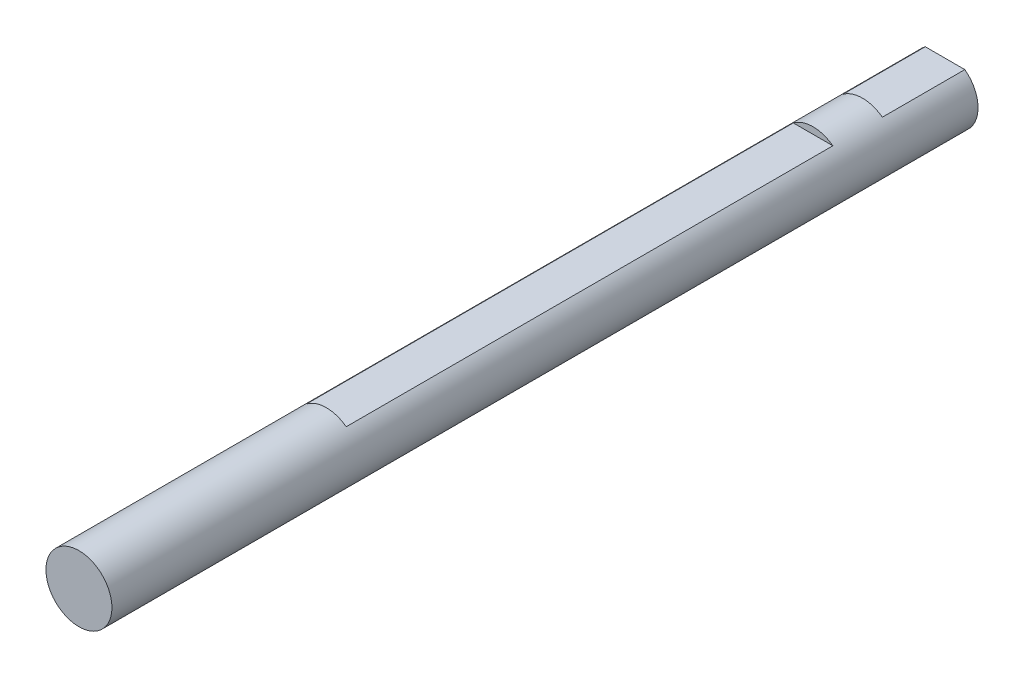
from build123d import *

# Parameters (mm, degrees)
SKETCH_1_R          = 4
EXTRUDE_1_DEPTH     = 105
CUT_EXTRUDE_1_DEPTH = 10
CUT_EXTRUDE_2_DEPTH = 59


with BuildPart() as part:
    # 草图1 → 凸台-拉伸1 (new body)
    with BuildSketch(Plane.XY):
        with Locations((-9.495904584, 0)):
            Circle(SKETCH_1_R)
    extrude(amount=EXTRUDE_1_DEPTH)

    # 草图2 → 切除-拉伸1 (cut)
    with BuildSketch(Plane(origin=(0, 0, 0), x_dir=(-1, 0, 0), z_dir=(0, 0, -1))):
        with BuildLine():
            Line((7.095904584, 3.2), (11.895904584, 3.2))
            ThreePointArc((11.895904584, 3.2), (9.495904584, 4), (7.095904584, 3.2))
        make_face()
    extrude(amount=-CUT_EXTRUDE_1_DEPTH, mode=Mode.SUBTRACT)

    # 草图3 → 切除-拉伸2 (cut)
    with BuildSketch(Plane(origin=(0, 0, 16), x_dir=(-1, 0, 0), z_dir=(0, 0, -1))):
        with BuildLine():
            Line((7.095904584, 3.2), (11.895904584, 3.2))
            ThreePointArc((11.895904584, 3.2), (9.495904584, 4), (7.095904584, 3.2))
        make_face()
    extrude(amount=-CUT_EXTRUDE_2_DEPTH, mode=Mode.SUBTRACT)


solid = part.part
